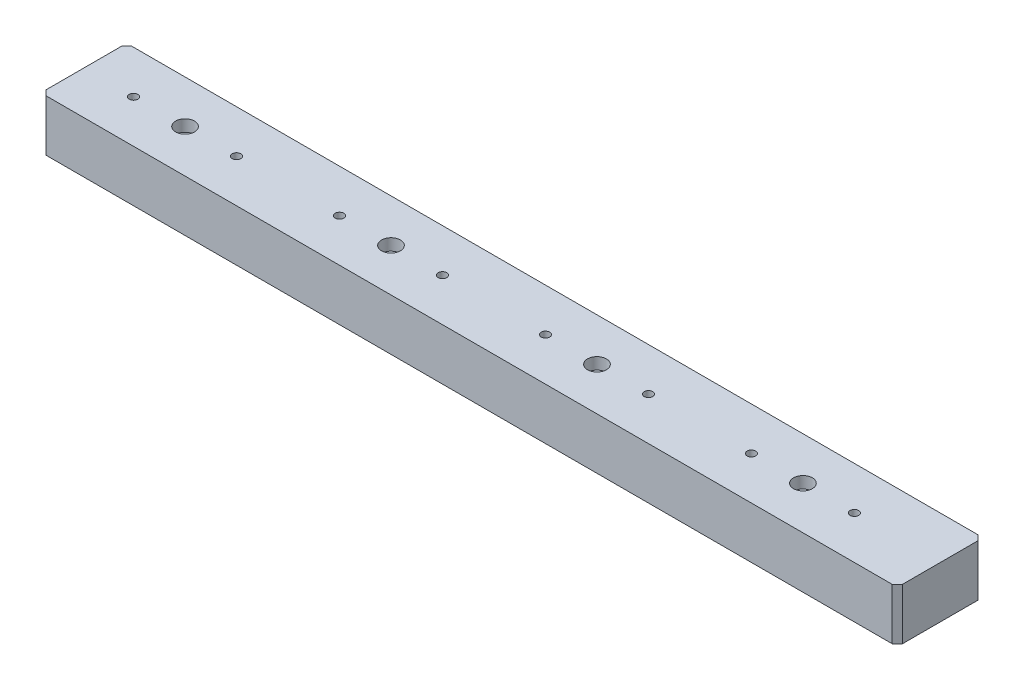
SolidWorks part; units mm, degrees
material "A6061 T6"
ref_plane "前视基准面" through (0, 0, 0) normal (0, 0, 1) x (1, 0, 0)
ref_plane "上视基准面" through (0, 0, 0) normal (0, 1, 0) x (1, 0, 0)
ref_plane "右视基准面" through (0, 0, 0) normal (1, 0, 0) x (0, 0, -1)
sketch "草图1" plane through (0, 0, 0) normal (0, 1, 0) x (1, 0, 0)
  line L1 (-249.5, 25) -> (249.5, 25)
  line L2 (-249.5, 25) -> (-249.5, -25)
  line L3 (-249.5, -25) -> (249.5, -25)
  line L4 (249.5, 25) -> (249.5, -25)
  line L5 (-249.5, 25) -> (249.5, -25) construction
  line L6 (-249.5, -25) -> (249.5, 25) construction
  point P0 (0, 0)
  dimension "D1" = 499
  dimension "D2" = 50
extrude "凸台-拉伸1" add sketch "草图1" along normal blind 30
chamfer "倒角1" distance 3 angle 45 4 edges at (249.5, 15, -25) (249.5, 15, 25) (-249.5, 15, 25) (-249.5, 15, -25)
hole_wizard "M6 螺纹孔1" positions "草图2" profile "草图3" tap size "M6" standard "GB"
sketch "草图2" plane through (0, 30, 0) normal (0, 1, 0) x (1, 0, 0)
  point P0 (199.5, 0)
  point P3 (139.5, 0)
  point P6 (79.5, 0)
  point P9 (19.5, 0)
  point P12 (-40.5, 0)
  point P15 (-100.5, 0)
  point P18 (-160.5, 0)
  point P21 (-220.5, 0)
sketch "草图3" plane through (199.5, 30, 0) normal (1, 0, 0) x (0, 0, 1)
  line L0 (0, 0) -> (0, 16.5022)
  line L1 (0, 16.5022) -> (2.5, 15)
  line L2 (2.5, 15) -> (2.5, 0)
  line L5 (2.5, 0) -> (0, 0)
  line L10 (0, 16.5022) -> (-2.5, 15) construction
  line L11 (0, -6.35) -> (0, 107.95) construction
  dimension "螺纹孔钻头直径" = 5
  dimension "螺纹孔钻头深度" = 15
  dimension "导头角度" = 118
cosmetic thread "孔螺蚊线1"
cosmetic thread "孔螺蚊线2"
cosmetic thread "孔螺蚊线3"
cosmetic thread "孔螺蚊线4"
cosmetic thread "孔螺蚊线5"
cosmetic thread "孔螺蚊线6"
cosmetic thread "孔螺蚊线7"
cosmetic thread "孔螺蚊线8"
hole_wizard "打孔尺寸(%根据)内六角圆柱头螺钉的类型1" positions "草图4" profile "草图5" counterbore size "M6" standard "GB"
sketch "草图4" plane through (0, 30, 0) normal (0, 1, 0) x (1, 0, 0)
  line L0 (249.5, -22) -> (249.5, 22) construction
  line L1 (-246.5, -25) -> (246.5, -25) construction
  point P0 (169.5, 0)
  point P2 (49.5, 0)
  point P4 (-70.5, 0)
  point P6 (-190.5, 0)
  dimension "D1" = 80
  dimension "D2" = 120
  dimension "D3" = 120
  dimension "D4" = 120
  dimension "D5" = 25
sketch "草图5" plane through (169.5, 30, 0) normal (1, 0, 0) x (0, 0, 1)
  line L0 (0, 0) -> (0, 31.9828)
  line L1 (0, 31.9828) -> (3.3, 30)
  line L2 (3.3, 30) -> (3.3, 6.8)
  line L3 (3.3, 6.8) -> (5.5, 6.8)
  line L4 (5.5, 6.8) -> (5.5, 0)
  line L5 (5.5, 0) -> (0, 0)
  line L10 (0, 31.9828) -> (-3.3, 30) construction
  line L11 (0, -6.35) -> (0, 107.95) construction
  dimension "孔直径" = 6.6
  dimension "孔深度" = 30
  dimension "柱形沉头孔直径" = 11
  dimension "柱形沉头孔深度" = 6.8
  dimension "导头角度" = 118
